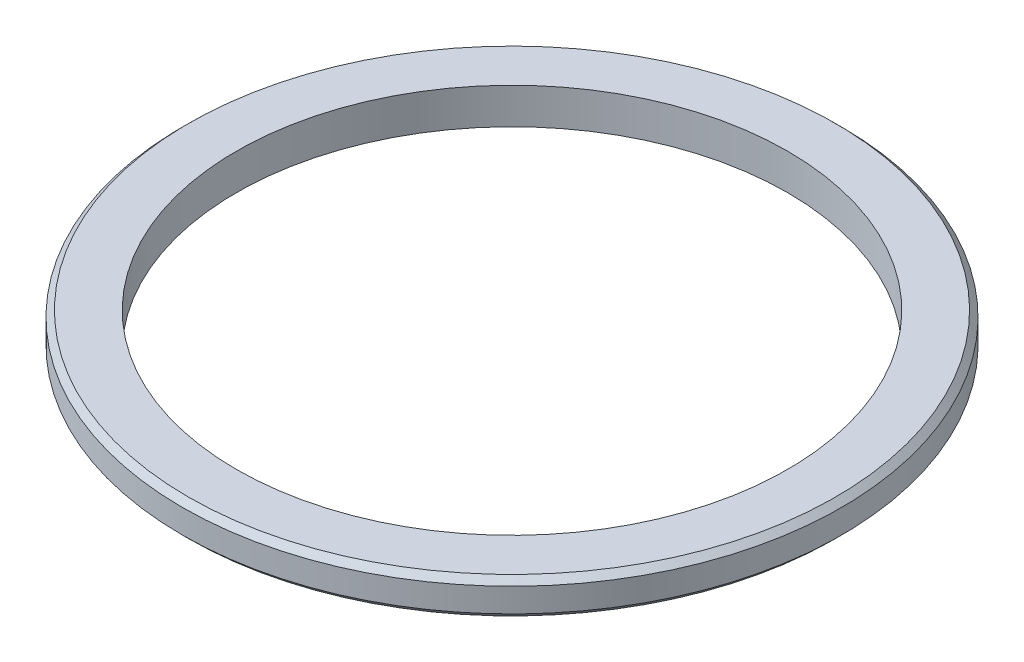
SolidWorks part; units mm, degrees
ref_plane "Front Plane" through (0, 0, 0) normal (0, 0, 1) x (1, 0, 0)
ref_plane "Top Plane" through (0, 0, 0) normal (0, 1, 0) x (1, 0, 0)
ref_plane "Right Plane" through (0, 0, 0) normal (1, 0, 0) x (0, 0, -1)
sketch "Sketch1" plane through (0, 0, 0) normal (0, 1, 0) x (1, 0, 0)
  circle A0 centre (0, 0) radius 27.5
  circle A1 centre (0, 0) radius 23
  dimension "D1" = 55
  dimension "D2" = 46
extrude "Boss-Extrude1" add sketch "Sketch1" along normal blind 3
chamfer "Chamfer1" distance 0.5 angle 45 2 edges at (0, 0, 27.5) (0, 3, 27.5)
